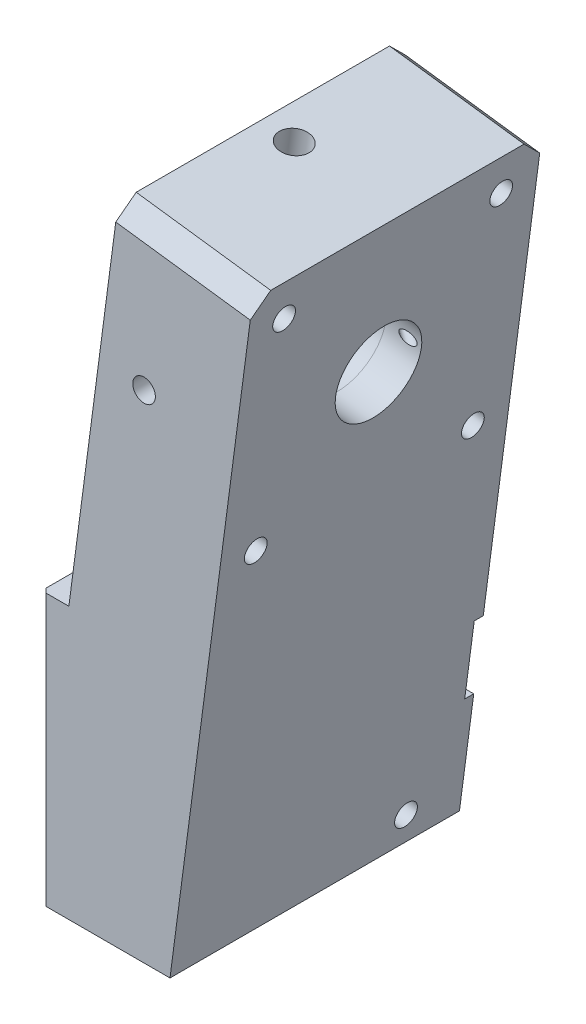
from build123d import *

# Parameters (mm, degrees)
BOSS_EXTRUDE1_DEPTH    = 16
SKETCH2_R              = 4.75
CUT_EXTRUDE1_DEPTH     = 77.207895426
CHAMFER1_SIZE          = 2
SKETCH3_R              = 7
CUT_EXTRUDE2_DEPTH     = 7
CHAMFER2_SIZE          = 4
CHAMFER2_SIZE2         = 0.3
M3_TAPPED_HOLE2_D      = 2.5
M3_TAPPED_HOLE2_DEPTH  = 7.5
M3_TAPPED_HOLE2_TIP    = 0.751075774
M4_TAPPED_HOLE1_D      = 3.3
M4_TAPPED_HOLE1_DEPTH  = 10.1
M4_TAPPED_HOLE1_TIP    = 0.991420021
CHAMFER3_SIZE          = 0.5
M4_TAPPED_HOLE3_REACH  = 76.329
M4_TAPPED_HOLE3_BORE_R = 1.65
M3_TAPPED_HOLE3_D      = 2.5
M3_TAPPED_HOLE3_DEPTH  = 8.5
M3_TAPPED_HOLE3_TIP    = 0.751075774
M3_TAPPED_HOLE4_D      = 2.5
M3_TAPPED_HOLE4_DEPTH  = 8.5
M3_TAPPED_HOLE4_TIP    = 0.751075774
SKETCH20_W             = 20
SKETCH20_H             = 8
CUT_EXTRUDE3_DEPTH     = 1
M3_TAPPED_HOLE5_D      = 2.5
M3_TAPPED_HOLE5_DEPTH  = 8.5
M3_TAPPED_HOLE5_TIP    = 0.751075774


with BuildPart() as part:
    # Sketch1 → Boss-Extrude1 (new, symmetric)
    with BuildSketch(Plane.XY):
        Polygon((0, 0), (0, 30), (3, 30), (8.445020016, 71.359033179), (23.316692936, 69.401140296), (14.179859481, 0), align=None)
    extrude(amount=BOSS_EXTRUDE1_DEPTH, both=True)

    # Sketch2 → Cut-Extrude1 (cut, through all)
    with BuildSketch(Plane(origin=(13.938275984, -1.835008845, 0), x_dir=(0, 0, -1), z_dir=(0.9914448613738108, -0.1305261922200488, 0))):
        with Locations(Location((0, 55.850843064, 0), (0, 0, 90))):
            Circle(SKETCH2_R)
    extrude(amount=-CUT_EXTRUDE1_DEPTH, mode=Mode.SUBTRACT)

    # Chamfer1
    chamfer1_edges = [part.edges().sort_by_distance(p)[0] for p in [
        (15.880856476, 70.380086738, 16),
        (15.880856476, 70.380086738, -16),
    ]]
    chamfer(chamfer1_edges, length=CHAMFER1_SIZE)

    # Sketch3 → Cut-Extrude2 (cut)
    with BuildSketch(Plane(origin=(-0.933396937, 0.122884038, 0), x_dir=(0, 0, 1), z_dir=(-0.9914448613738109, 0.13052619222004871, 0))):
        with Locations(Location((0, 55.850843064, 0), (0, 0, 270))):
            Circle(SKETCH3_R)
    extrude(amount=-CUT_EXTRUDE2_DEPTH, mode=Mode.SUBTRACT)

    # Sketch4 → M3 Tapped Hole1 (revolve, cut)
    with BuildSketch(Plane(origin=(11.313825247, 54.843284436, 16), x_dir=(0, -1, 0), z_dir=(1, 0, 0))):
        Polygon((0, 0), (0, 7.251075774), (1.25, 6.5), (1.25, 0), align=None)
    m3_tapped_hole1 = revolve(axis=Axis((11.313825247, 54.843284436, 22.35), (0, 0, -1)), mode=Mode.SUBTRACT)

    # Sketch6 → Cut-Revolve1 (revolve, cut)
    with BuildSketch(Plane(origin=(7.289997877, 55.373031359, 0), x_dir=(0.9914448613738107, -0.1305261922200494, 0), z_dir=(0.1305261922200494, 0.9914448613738107, 0)), mode=Mode.PRIVATE) as cut_revolve1_sk:
        Polygon((4.058548818, -10.905172414), (14.587796398, -3.280544856), (14.939702285, -3.766510129), (4.410454705, -11.391137687), align=None)
    cut_revolve1 = revolve(cut_revolve1_sk.sketch.rotate(Axis((12.553131324, 54.680126696, 10), (0.80301295441403, -0.10571866104363936, -0.5865098121518437)), 355.584640013), axis=Axis((12.553131324, 54.680126696, 10), (0.80301295441403, -0.10571866104363936, -0.5865098121518437)), mode=Mode.SUBTRACT)

    # Mirror1: M3 Tapped Hole1, Cut-Revolve1 across plane
    add(m3_tapped_hole1.mirror(Plane.XY), mode=Mode.SUBTRACT)
    add(cut_revolve1.mirror(Plane.XY), mode=Mode.SUBTRACT)

    # Chamfer2
    chamfer2_edges = [part.edges().sort_by_distance(p)[0] for p in [
        (12.676715557, 49.87286896, 0),
    ]]
    chamfer2_side = [part.faces().sort_by_distance(p)[0] for p in [
        (16.642495002, 49.350764192, 0),
    ]]
    chamfer(chamfer2_edges, length=CHAMFER2_SIZE, length2=CHAMFER2_SIZE2, reference=chamfer2_side[0])

    # M3 Tapped Hole2
    with Locations(Plane(origin=(13.938275984, -1.835008845, 0), x_dir=(0, 0, -1), z_dir=(0.9914448613738107, -0.13052619222004877, 0))):
        with Locations((-12, 67.850843064), (12, 67.850843064), (12, 43.850843064), (-12, 43.850843064)):
            Hole(M3_TAPPED_HOLE2_D / 2, depth=M3_TAPPED_HOLE2_DEPTH)
            with Locations((0, 0, -(M3_TAPPED_HOLE2_DEPTH + M3_TAPPED_HOLE2_TIP / 2))):  # 118° drill point
                Cone(0, M3_TAPPED_HOLE2_D / 2, M3_TAPPED_HOLE2_TIP, mode=Mode.SUBTRACT)

    # M4 Tapped Hole1
    with Locations(Plane.ZY):
        with Locations((-9, 23), (9, 23), (9, 7), (-9, 7)):
            Hole(M4_TAPPED_HOLE1_D / 2, depth=M4_TAPPED_HOLE1_DEPTH)
            with Locations((0, 0, -(M4_TAPPED_HOLE1_DEPTH + M4_TAPPED_HOLE1_TIP / 2))):  # 118° drill point
                Cone(0, M4_TAPPED_HOLE1_D / 2, M4_TAPPED_HOLE1_TIP, mode=Mode.SUBTRACT)

    # Chamfer3
    chamfer3_edges = [part.edges().sort_by_distance(p)[0] for p in [
        (0, 15, 16),
        (0, 15, -16),
    ]]
    chamfer(chamfer3_edges, length=CHAMFER3_SIZE)

    # M4 Tapped Hole3 bore → M4 Tapped Hole3 (cut, up to next)
    with BuildSketch(Plane(origin=(9.378416953, 71.236149141, 0), x_dir=(0.9914448613738107, -0.1305261922200494, 0), z_dir=(0.1305261922200494, 0.9914448613738107, 0)), mode=Mode.PRIVATE) as m4_tapped_hole3_sk1:
        with Locations((2.558548818, 0)):
            Circle(M4_TAPPED_HOLE3_BORE_R)
    m4_tapped_hole3_tool1 = extrude(m4_tapped_hole3_sk1.sketch, amount=-M4_TAPPED_HOLE3_REACH, mode=Mode.PRIVATE) & part.part
    add(m4_tapped_hole3_tool1.solids().sort_by_distance((11.915077, 70.902192, 0))[0], mode=Mode.SUBTRACT)

    # M3 Tapped Hole3
    with Locations(Plane(origin=(13.938275984, -1.835008845, 0), x_dir=(0, 0, -1), z_dir=(0.9914448613738108, -0.1305261922200488, 0))):
        with Locations((9.7, 4.850843064)):
            Hole(M3_TAPPED_HOLE3_D / 2, depth=M3_TAPPED_HOLE3_DEPTH)
            with Locations((0, 0, -(M3_TAPPED_HOLE3_DEPTH + M3_TAPPED_HOLE3_TIP / 2))):  # 118° drill point
                Cone(0, M3_TAPPED_HOLE3_D / 2, M3_TAPPED_HOLE3_TIP, mode=Mode.SUBTRACT)

    # M3 Tapped Hole4
    with Locations(Plane(origin=(0, 0, -16), x_dir=(-1, 0, 0), z_dir=(0, 0, -1))):
        with Locations((-15.788403885, 36), (-7.788403885, 36)):
            Hole(M3_TAPPED_HOLE4_D / 2, depth=M3_TAPPED_HOLE4_DEPTH)
            with Locations((0, 0, -(M3_TAPPED_HOLE4_DEPTH + M3_TAPPED_HOLE4_TIP / 2))):  # 118° drill point
                Cone(0, M3_TAPPED_HOLE4_D / 2, M3_TAPPED_HOLE4_TIP, mode=Mode.SUBTRACT)

    # Sketch20 → Cut-Extrude3 (cut)
    with BuildSketch(Plane(origin=(0, 0, -16), x_dir=(-1, 0, 0), z_dir=(0, 0, -1))):
        with Locations((-10, 16)):
            Rectangle(SKETCH20_W, SKETCH20_H)
    extrude(amount=-CUT_EXTRUDE3_DEPTH, mode=Mode.SUBTRACT)

    # M3 Tapped Hole5
    with Locations(Plane(origin=(0, 0, -15), x_dir=(-1, 0, 0), z_dir=(0, 0, -1))):
        with Locations((-13, 16), (-6, 16)):
            Hole(M3_TAPPED_HOLE5_D / 2, depth=M3_TAPPED_HOLE5_DEPTH)
            with Locations((0, 0, -(M3_TAPPED_HOLE5_DEPTH + M3_TAPPED_HOLE5_TIP / 2))):  # 118° drill point
                Cone(0, M3_TAPPED_HOLE5_D / 2, M3_TAPPED_HOLE5_TIP, mode=Mode.SUBTRACT)


solid = part.part
